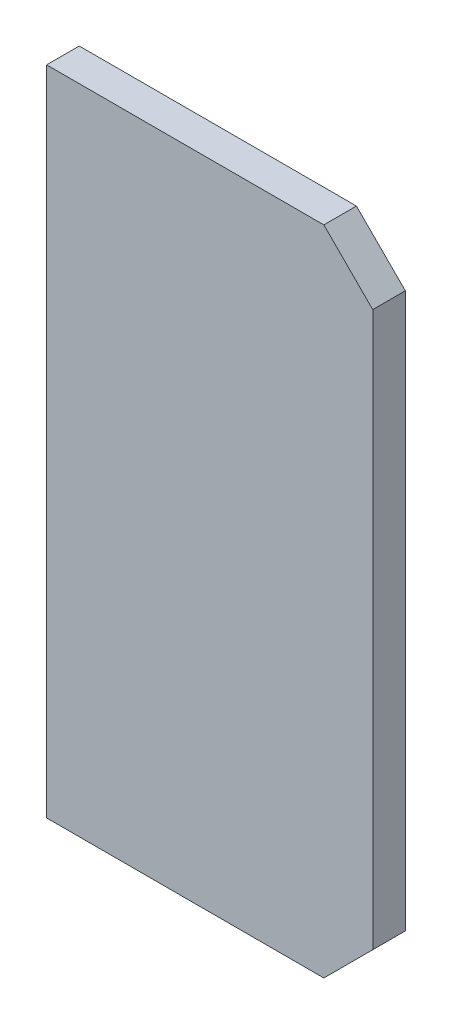
from build123d import *

# Parameters (mm, degrees)
EXTRUDE_1_DEPTH = 5
CHAMFER_1_SIZE  = 15
EXTRUDE_2_DEPTH = 10


with BuildPart() as part:
    # 草图1 → 凸台-拉伸1 (new, symmetric)
    with BuildSketch(Plane.XY):
        Polygon((0, 0), (0, 150), (46, 200), (100, 200), (100, 0), align=None)
    extrude(amount=EXTRUDE_1_DEPTH, both=True)

    # 倒角1
    chamfer_1_edges = [part.edges().sort_by_distance(p)[0] for p in [
        (100, 200, 0),
        (100, 0, 0),
    ]]
    chamfer(chamfer_1_edges, length=CHAMFER_1_SIZE)

    # 草图2 → 凸台-拉伸2 (add)
    with BuildSketch(Plane.XY.offset(5)):
        Polygon((0, 150), (0, 200), (46, 200), align=None)
    extrude(amount=-EXTRUDE_2_DEPTH)


solid = part.part
